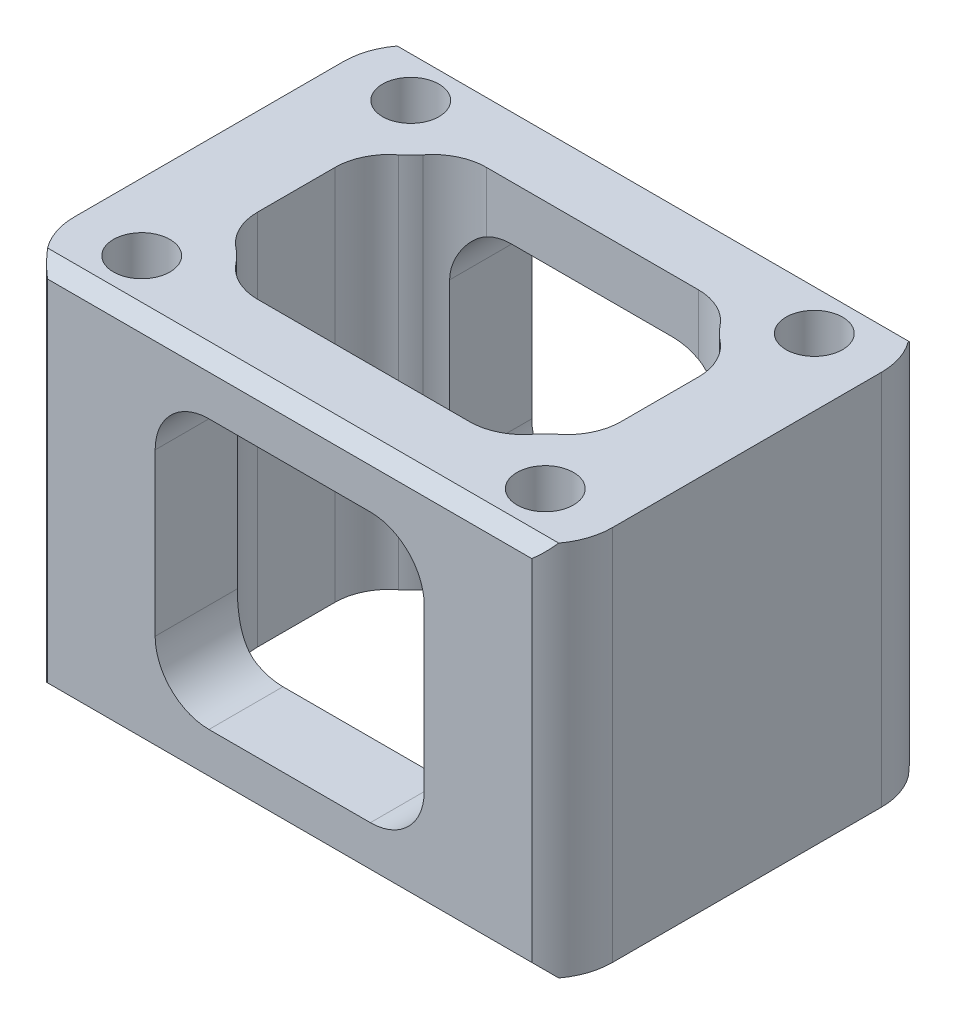
SolidWorks part; units mm, degrees
material "ABS"
ref_plane "前视基准面" through (0, 0, 0) normal (0, 0, 1) x (1, 0, 0)
ref_plane "上视基准面" through (0, 0, 0) normal (0, 1, 0) x (1, 0, 0)
ref_plane "右视基准面" through (0, 0, 0) normal (1, 0, 0) x (0, 0, -1)
other "Configuration Table"
sketch "草图1" plane through (0, 0, 0) normal (0, 1, 0) x (1, 0, 0)
  line L1 (-20, -14) -> (20, -14)
  line L2 (-20, -14) -> (-20, 14)
  line L3 (-20, 14) -> (20, 14)
  line L4 (20, -14) -> (20, 14)
  line L5 (-20, -14) -> (20, 14) construction
  line L6 (-20, 14) -> (20, -14) construction
  point P0 (0, 0)
  dimension "D1" = 28
  dimension "D2" = 40
extrude "凸台-拉伸1" add sketch "草图1" along normal blind 28
sketch "草图2" plane through (0, 28, 0) normal (0, 1, 0) x (1, 0, 0)
  line L0 (-15, 0) -> (0, 0) construction
  line L1 (0, 0) -> (0, 10) construction
  line L12 (15, -10) -> (15, 10) construction
  line L13 (15, 10) -> (-15, 10) construction
  line L14 (-15, 10) -> (-15, -10) construction
  line L15 (-15, -10) -> (15, -10) construction
  circle A0 centre (-15, 10) radius 2.1
  circle A1 centre (-15, -10) radius 2.1
  circle A2 centre (15, -10) radius 2.1
  circle A3 centre (15, 10) radius 2.1
  circle A4 centre (-15, 10) radius 4.05 construction
  circle A5 centre (-15, -10) radius 4.05 construction
  circle A6 centre (15, -10) radius 4.05 construction
  circle A7 centre (15, 10) radius 4.05 construction
  dimension "D2" = 4.2
  dimension "D1" = 30
  dimension "D4" = 20
  dimension "D3" = 1.95
extrude "切除-拉伸1" cut sketch "草图2" against normal through all
sketch "草图3" plane through (0, 28, 0) normal (0, 1, 0) x (1, 0, 0)
  line L1 (-15, -10) -> (15, -10) construction
  line L2 (-15, -10) -> (-15, 10) construction
  line L3 (-15, 10) -> (15, 10) construction
  line L4 (15, -10) -> (15, 10) construction
  line L8 (-13.5, -5.2303) -> (-13.5, 5.2303)
  line L9 (-10.2303, 8.5) -> (10.2303, 8.5)
  line L10 (13.5, -5.2303) -> (13.5, 5.2303)
  line L11 (-10.2303, -8.5) -> (10.2303, -8.5)
  line L14 (-13.5, 8.5) -> (13.5, 8.5) construction
  line L15 (-13.5, -8.5) -> (-13.5, 8.5) construction
  line L16 (13.5, -8.5) -> (13.5, 8.5) construction
  line L18 (-13.5, -8.5) -> (13.5, -8.5) construction
  line L24 (20, -14) -> (20, 14)
  line L25 (20, 14) -> (-20, 14)
  line L26 (-20, 14) -> (-20, -14)
  line L27 (-20, -14) -> (20, -14)
  line L28 (20, -10) -> (20, 10)
  line L29 (12, 14) -> (-18, 14)
  line L30 (-20, 10) -> (-20, -10)
  line L31 (-12, -14) -> (18, -14)
  arc A0 (-13.5, 5.2303) -> (-10.2303, 8.5) centre (-15, 10) ccw
  arc A1 (-10.2303, -8.5) -> (-13.5, -5.2303) centre (-15, -10) ccw
  arc A2 (13.5, -5.2303) -> (10.2303, -8.5) centre (15, -10) ccw
  arc A3 (20, 10) -> (12, 14) centre (15, 10) ccw
  arc A4 (-18, 14) -> (-20, 10) centre (-15, 10) ccw
  arc A5 (10.2303, 8.5) -> (13.5, 5.2303) centre (15, 10) ccw
  arc A6 (18, -14) -> (20, -10) centre (15, -10) ccw
  arc A7 (-20, -10) -> (-12, -14) centre (-15, -10) ccw
  dimension "D1" = 10
  dimension "D3" = 1.5
  dimension "D4" = 0
extrude "切除-拉伸2" cut sketch "草图3" against normal through all flip side to cut
fillet "圆角3" radius 4 8 edges at (-10.2303, 14, -8.5) (10.2303, 14, -8.5) (13.5, 14, -5.2303) (13.5, 14, 5.2303) (10.2303, 14, 8.5) (-10.2303, 14, 8.5) (-13.5, 14, 5.2303) (-13.5, 14, -5.2303)
sketch "草图6" plane through (0, 0, 14) normal (0, 0, 1) x (1, 0, 0)
  line L0 (-18, 0) -> (18, 0) construction
  line L1 (-10, 4) -> (10, 4)
  line L2 (-10, 4) -> (-10, 24)
  line L3 (-10, 24) -> (10, 24)
  line L4 (10, 4) -> (10, 24)
  line L5 (-18, 28) -> (18, 28) construction
  point P4 (0, 4)
  dimension "D1" = 20
  dimension "D2" = 4
  dimension "D3" = 4
extrude "切除-拉伸4" cut sketch "草图6" against normal through all
fillet "圆角4" radius 4 8 edges at (10, 4, -10.9448) (-10, 4, -10.9448) (-10, 24, -10.9448) (10, 24, -10.9448) (10, 4, 10.9448) (-10, 4, 10.9448) (-10, 24, 10.9448) (10, 24, 10.9448)
chamfer "倒角1" distance 1 angle 45 4 edges at (0, 28, -14) (0, 0, -14) (0, 0, 14) (0, 28, 14)
